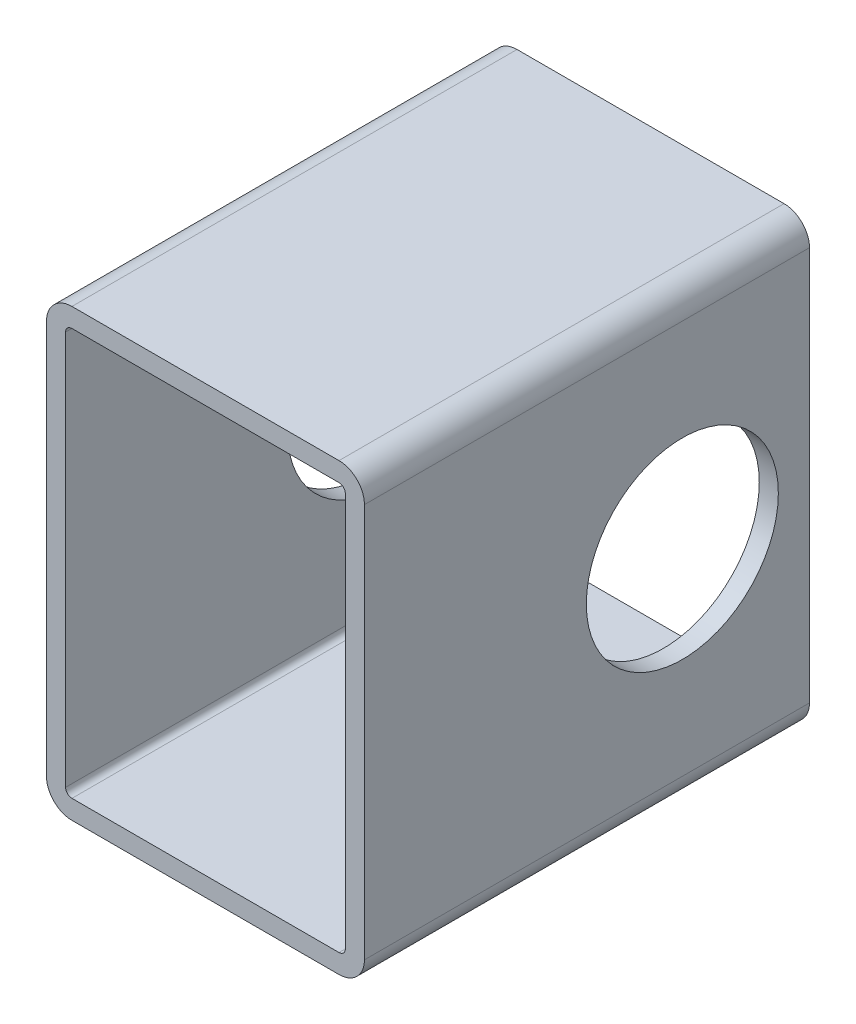
from build123d import *

# Parameters (mm, degrees)
EXTRUDE_THIN1_DEPTH = 70
SKETCH2_R           = 15.1
CUT_EXTRUDE1_DEPTH  = 93.870878105


with BuildPart() as part:
    # Sketch1 → Extrude-Thin1 (new body)
    with BuildSketch(Plane.XY):
        with BuildLine():
            Line((-25, 31), (-25, -31))
            ThreePointArc((-25, -31), (-23.828427125, -33.828427125), (-21, -35))
            Line((-21, -35), (21, -35))
            ThreePointArc((21, -35), (23.828427125, -33.828427125), (25, -31))
            Line((25, -31), (25, 31))
            ThreePointArc((25, 31), (23.828427125, 33.828427125), (21, 35))
            Line((21, 35), (-21, 35))
            ThreePointArc((-21, 35), (-23.828427125, 33.828427125), (-25, 31))
        make_face()
        with BuildLine():
            Line((-22, 31), (-22, -31))
            ThreePointArc((-22, -31), (-21.707106781, -31.707106781), (-21, -32))
            Line((-21, -32), (21, -32))
            ThreePointArc((21, -32), (21.707106781, -31.707106781), (22, -31))
            Line((22, -31), (22, 31))
            ThreePointArc((22, 31), (21.707106781, 31.707106781), (21, 32))
            Line((21, 32), (-21, 32))
            ThreePointArc((-21, 32), (-21.707106781, 31.707106781), (-22, 31))
        make_face(mode=Mode.SUBTRACT)
    extrude(amount=EXTRUDE_THIN1_DEPTH)

    # Sketch2 → Cut-Extrude1 (cut, through all)
    with BuildSketch(Plane(origin=(25, 0, 0), x_dir=(0, 0, -1), z_dir=(1, 0, 0))):
        with Locations((-20, 0)):
            Circle(SKETCH2_R)
    extrude(amount=-CUT_EXTRUDE1_DEPTH, mode=Mode.SUBTRACT)


solid = part.part
